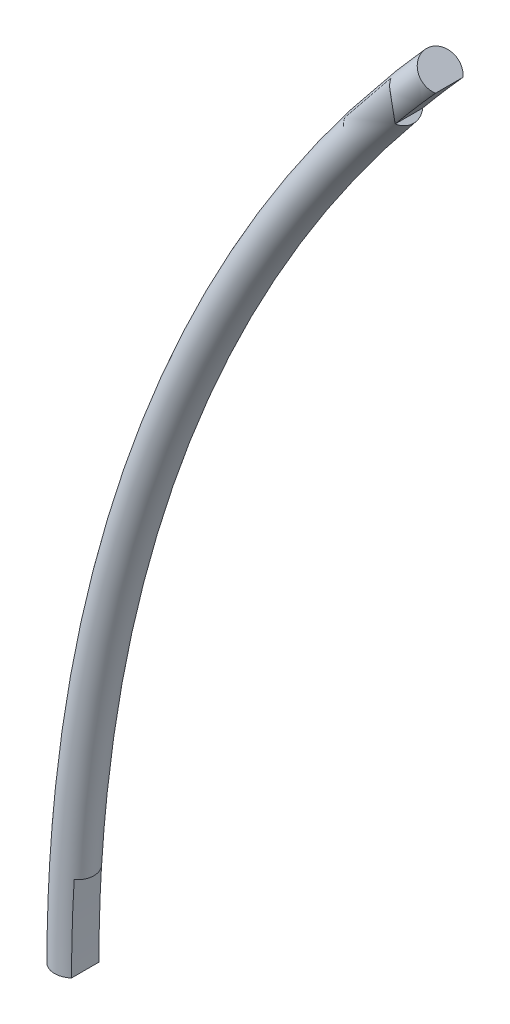
from build123d import *

# Parameters (mm, degrees)
SWEEP1_PROFILE_R   = 3
CUT_EXTRUDE1_DEPTH = 25


with BuildPart() as part:
    # Sweep1: sweep along a path in Sketch1
    with BuildLine(Plane.XY) as sweep1_path:
        ThreePointArc((-173.152744336, 155.907431282), (-217.524239374, 83.499732244), (-233, 0))
    # Sweep1 profile (on start of the path) → Sweep1 (sweep)
    with BuildSketch(Plane(origin=(-173.152744336, 155.907431282, 0), x_dir=(-0.7431448254773938, 0.6691306063588589, 0), z_dir=(-0.6691306063588589, -0.7431448254773938, 0))):
        Circle(SWEEP1_PROFILE_R)
    sweep(path=sweep1_path.line)

    # Sketch6 → Cut-Extrude1 (cut, symmetric)
    with BuildSketch(Plane.XY):
        with BuildLine():
            Line((0, 0), (-230.569138435, 14.102212633))
            ThreePointArc((-230.569138435, 14.102212633), (-230.892259483, 7.054396551), (-231, 0))
            Line((-231, 0), (0, 0))
        make_face()
        with BuildLine():
            Line((0, 0), (-171.666454685, 154.569170069))
            ThreePointArc((-171.666454685, 154.569170069), (-174.997511393, 150.787502819), (-178.245278763, 146.934068884))
            Line((-178.245278763, 146.934068884), (0, 0))
        make_face()
    extrude(amount=CUT_EXTRUDE1_DEPTH, both=True, mode=Mode.SUBTRACT)


solid = part.part
